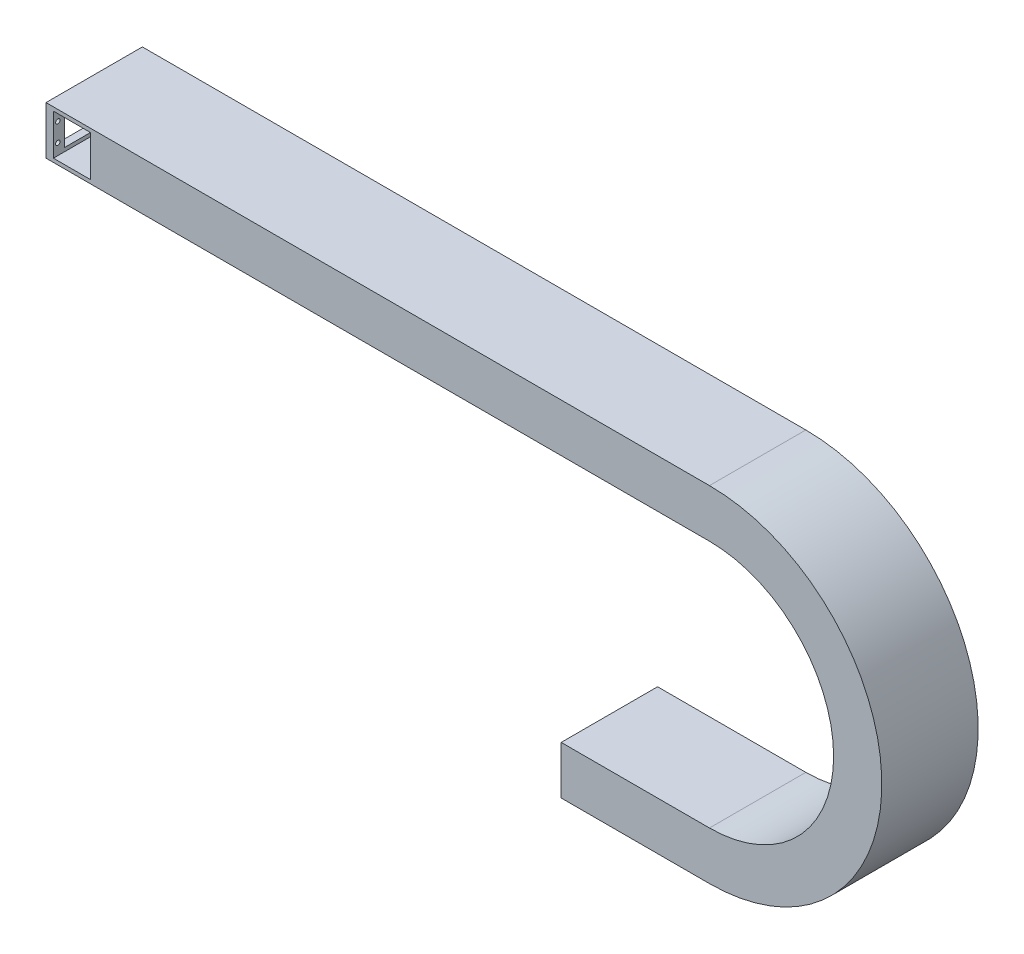
SolidWorks part; units mm, degrees
ref_plane "前视基准面" through (0, 0, 0) normal (0, 0, 1) x (1, 0, 0)
ref_plane "上视基准面" through (0, 0, 0) normal (0, 1, 0) x (1, 0, 0)
ref_plane "右视基准面" through (0, 0, 0) normal (1, 0, 0) x (0, 0, -1)
sketch "草图1" plane through (0, 0, 0) normal (0, 0, 1) x (1, 0, 0)
  line L0 (-5035.4277, 234.0221) -> (-5930.4277, 234.0221)
  line L1 (-5035.4277, -100.9779) -> (-5235.4277, -100.9779)
  line L2 (-5035.4277, -165.9779) -> (-5235.4277, -165.9779)
  line L3 (-5035.4277, 299.0221) -> (-5930.4277, 299.0221)
  line L4 (-5930.4277, 299.0221) -> (-5930.4277, 234.0221)
  line L5 (-5235.4277, -165.9779) -> (-5235.4277, -100.9779)
  arc A0 (-5035.4277, -100.9779) -> (-5035.4277, 234.0221) centre (-5035.4277, 66.5221) ccw
  arc A1 (-5035.4277, -165.9779) -> (-5035.4277, 299.0221) centre (-5035.4277, 66.5221) ccw
  dimension "D1" = 895
  dimension "D4" = 167.5
  dimension "D2" = 200
  dimension "D3" = 65
extrude "凸台-拉伸1" add sketch "草图1" along normal blind 130
sketch "草图2" plane through (-5930.4277, 0, 0) normal (-1, 0, 0) x (0, 0, 1)
  line L0 (130, 299.0221) -> (0, 299.0221) construction
  line L1 (130, 299.0221) -> (130, 234.0221) construction
  circle A0 centre (6, 279.0221) radius 3
  circle A1 centre (6, 254.0221) radius 3
  circle A2 centre (124, 279.0221) radius 3
  circle A3 centre (124, 254.0221) radius 3
  dimension "D1" = 25
  dimension "D2" = 25
  dimension "D3" = 6
  dimension "D4" = 118
  dimension "D5" = 20
  dimension "D6" = 6
  dimension "D8" = 118
  dimension "D7" = 20
extrude "切除-拉伸1" cut sketch "草图2" against normal blind 20
sketch "草图9" plane through (0, 0, 130) normal (0, 0, 1) x (1, 0, 0)
  line L0 (-5035.4277, 299.0221) -> (-5930.4277, 299.0221) construction
  line L1 (-5920.4277, 294.0221) -> (-5870.4277, 294.0221)
  line L2 (-5920.4277, 294.0221) -> (-5920.4277, 239.0221)
  line L3 (-5920.4277, 239.0221) -> (-5870.4277, 239.0221)
  line L4 (-5870.4277, 294.0221) -> (-5870.4277, 239.0221)
  line L5 (-5930.4277, 234.0221) -> (-5035.4277, 234.0221) construction
  line L6 (-5930.4277, 299.0221) -> (-5930.4277, 234.0221) construction
  dimension "D1" = 5
  dimension "D2" = 5
  dimension "D3" = 10
  dimension "D4" = 50
extrude "切除-拉伸2" cut sketch "草图9" against normal blind 150
sketch "草图10" plane through (-5930.4277, 0, 0) normal (-1, 0, 0) x (0, 0, 1)
  line L0 (130, 299.0221) -> (0, 299.0221) construction
  line L1 (15, 289.0221) -> (115, 289.0221)
  line L2 (15, 289.0221) -> (15, 244.0221)
  line L3 (15, 244.0221) -> (115, 244.0221)
  line L4 (115, 289.0221) -> (115, 244.0221)
  line L5 (0, 299.0221) -> (0, 234.0221) construction
  dimension "D1" = 100
  dimension "D2" = 45
  dimension "D3" = 10
  dimension "D4" = 15
extrude "切除-拉伸3" cut sketch "草图10" against normal blind 200
